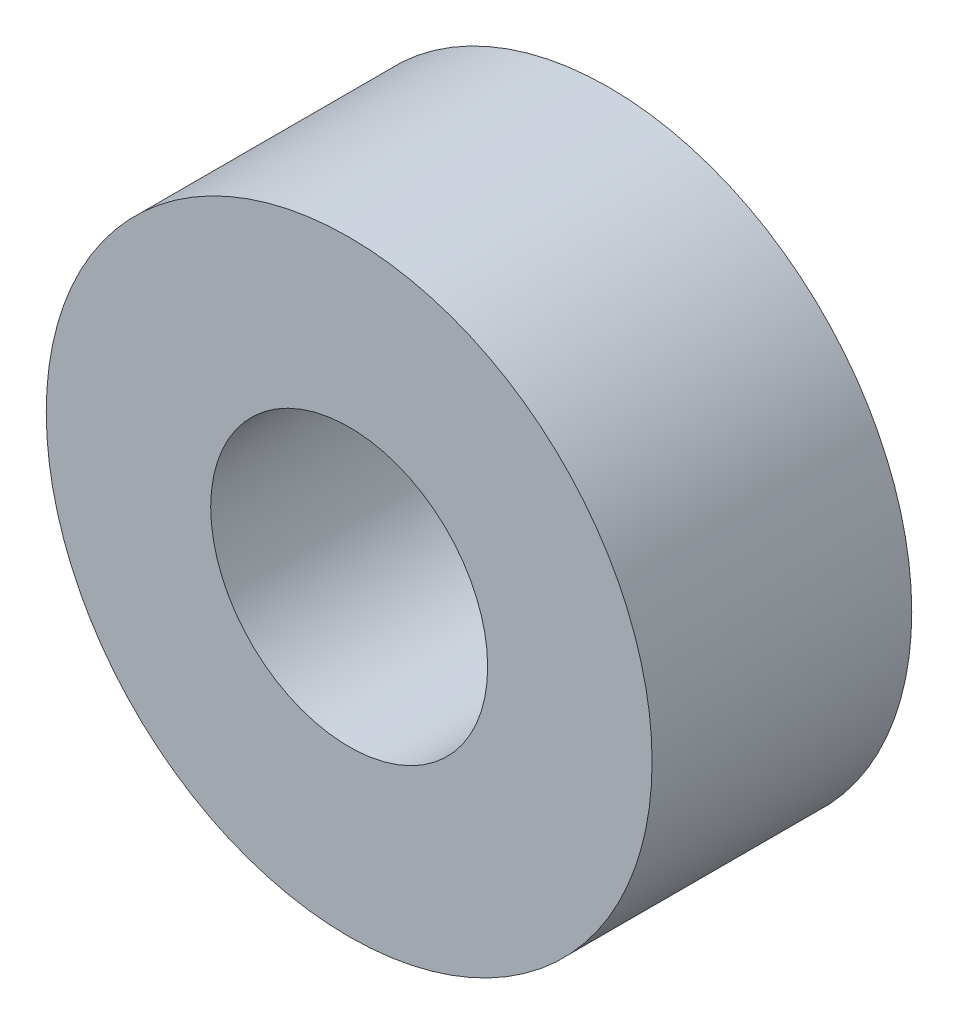
SolidWorks part; units mm, degrees
ref_plane "前视基准面" through (0, 0, 0) normal (0, 0, 1) x (1, 0, 0)
ref_plane "上视基准面" through (0, 0, 0) normal (0, 1, 0) x (1, 0, 0)
ref_plane "右视基准面" through (0, 0, 0) normal (1, 0, 0) x (0, 0, -1)
sketch "草图1" plane through (0, 0, 0) normal (0, 0, 1) x (1, 0, 0)
  circle A0 centre (0, 0) radius 8
  circle A1 centre (0, 0) radius 17.5
  dimension "D1" = 16
  dimension "D2" = 35
extrude "凸台-拉伸1" add sketch "草图1" along normal mid plane 15
